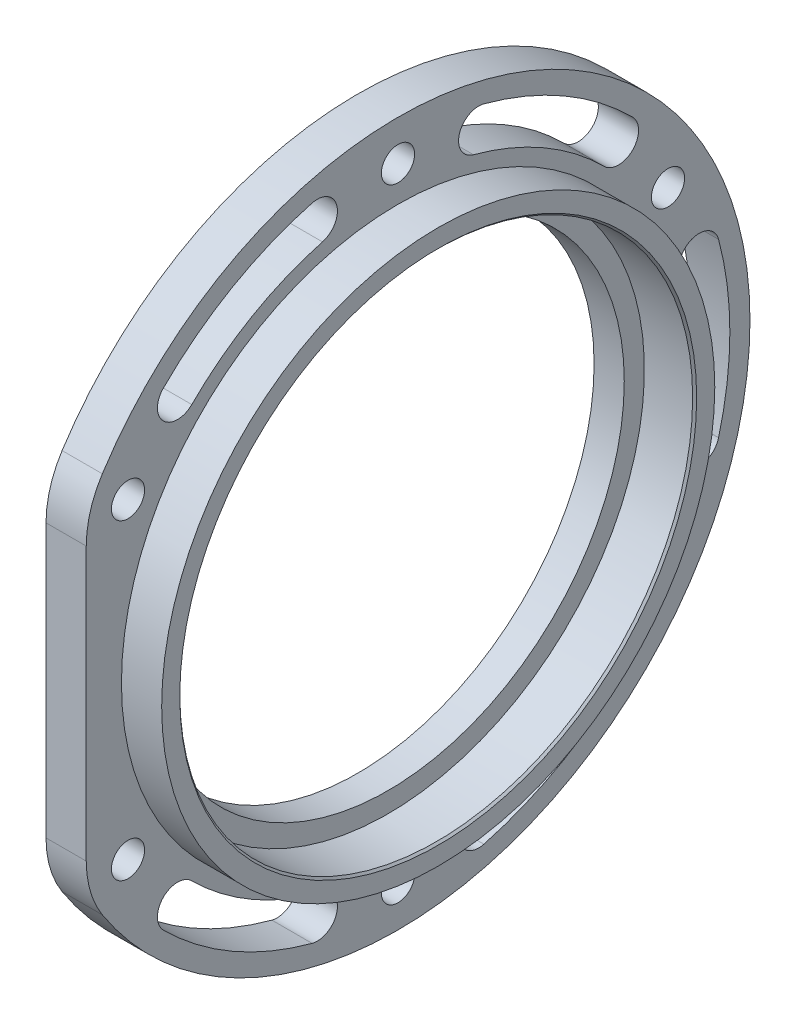
SolidWorks part; units mm, degrees
material "6061 合金"
ref_plane "前视基准面" through (0, 0, 0) normal (0, 0, 1) x (1, 0, 0)
ref_plane "上视基准面" through (0, 0, 0) normal (0, 1, 0) x (1, 0, 0)
ref_plane "右视基准面" through (0, 0, 0) normal (1, 0, 0) x (0, 0, -1)
other "Configuration Table"
sketch "草图1" plane through (0, 0, 0) normal (0, 1, 0) x (1, 0, 0)
  line L0 (-554.3921, 0) -> (27165.2107, 0) construction
  line L1 (0, 23.5) -> (0, 35)
  line L4 (0, 35) -> (4, 35)
  line L6 (8, 25.5) -> (3, 25.5)
  line L7 (3, 25.5) -> (3, 23.5)
  line L8 (3, 23.5) -> (0, 23.5)
  line L9 (4, 35) -> (4, 27.5)
  line L10 (4, 27.5) -> (8, 27.5)
  line L11 (8, 27.5) -> (8, 25.5)
  dimension "D1" = 47
  dimension "D2" = 51
  dimension "D3" = 5
  dimension "D4" = 4
  dimension "D6" = 70
  dimension "D7" = 3
  dimension "D9" = 55
revolve "旋转1" add sketch "草图1" angle 360 about L0
sketch "草图2" plane through (4, 0, 0) normal (1, 0, 0) x (0, 0, -1)
  circle A0 centre (0, 0) radius 31 construction
  point P3 (0, 31)
  point P6 (26.8468, 15.5)
  point P7 (26.8468, -15.5)
  point P8 (0, -31)
  point P9 (-26.8468, -15.5)
  point P10 (-26.8468, 15.5)
  point P11 (0, 0)
  dimension "D1" = 62
  dimension "D2" = 6
hole_wizard "M4 螺纹孔1" positions "草图2" profile "草图3" tap size "M4" standard "ISO" end condition through all
sketch "草图3" plane through (4, 0, 0) normal (0, 1, 0) x (0, 0, -1)
  line L0 (0, 0) -> (0, 4)
  line L1 (0, 4) -> (1.65, 4)
  line L2 (1.65, 4) -> (1.65, 0)
  line L5 (1.65, 0) -> (0, 0)
  line L11 (0, -6.35) -> (0, 107.95) construction
  dimension "通孔螺纹孔钻头直径" = 3.3
  dimension "通孔螺纹孔钻头深度" = 4
cosmetic thread "孔螺纹线1" parameters "D2"=4
cosmetic thread "孔螺纹线2" parameters "D2"=4
cosmetic thread "孔螺纹线3" parameters "D2"=4
cosmetic thread "孔螺纹线4" parameters "D2"=4
cosmetic thread "孔螺纹线5" parameters "D2"=4
cosmetic thread "孔螺纹线6" parameters "D2"=4
sketch "草图4" plane through (4, 0, 0) normal (1, 0, 0) x (0, 0, -1)
  line L0 (-31, -16.2481) -> (-31, 16.2481)
  line L1 (-26.8468, 15.5) -> (-26.8468, -15.5) construction
  circle A0 centre (0, 0) radius 35 construction
  circle A2 centre (0, 0) radius 35
  arc A3 (-31, 16.2481) -> (-31, -16.2481) centre (0, 0) ccw
  dimension "D1" = 31
  dimension "D2" = 0
extrude "切除-拉伸1" cut sketch "草图4" against normal blind 10
fillet "圆角1" radius 10 2 edges at (2, -16.2481, 31) (2, 16.2481, 31)
sketch "草图5" plane through (4, 0, 0) normal (1, 0, 0) x (0, 0, -1)
  line L0 (0, 31) -> (0, 0) construction
  line L1 (0, 0) -> (15.5, 26.8468) construction
  line L2 (8.0234, 29.9437) -> (0, 0) construction
  line L3 (0, 0) -> (21.9203, 21.9203) construction
  arc A0 (8.0234, 29.9437) -> (21.9203, 21.9203) centre (0, 0) cw construction
  arc A1 (23.3345, 23.3345) -> (8.541, 31.8756) centre (0, 0) ccw
  arc A2 (20.5061, 20.5061) -> (7.5058, 28.0118) centre (0, 0) ccw
  arc A3 (20.5061, 20.5061) -> (23.3345, 23.3345) centre (21.9203, 21.9203) ccw
  arc A4 (8.541, 31.8756) -> (7.5058, 28.0118) centre (8.0234, 29.9437) ccw
  arc A5 (29.9437, 8.0234) -> (29.9437, -8.0234) centre (0, 0) cw construction
  arc A6 (31.8756, -8.541) -> (31.8756, 8.541) centre (0, 0) ccw
  arc A7 (28.0118, -7.5058) -> (28.0118, 7.5058) centre (0, 0) ccw
  arc A8 (28.0118, -7.5058) -> (31.8756, -8.541) centre (29.9437, -8.0234) ccw
  arc A9 (31.8756, 8.541) -> (28.0118, 7.5058) centre (29.9437, 8.0234) ccw
  arc A10 (21.9203, -21.9203) -> (8.0234, -29.9437) centre (0, 0) cw construction
  arc A11 (8.541, -31.8756) -> (23.3345, -23.3345) centre (0, 0) ccw
  arc A12 (7.5058, -28.0118) -> (20.5061, -20.5061) centre (0, 0) ccw
  arc A13 (7.5058, -28.0118) -> (8.541, -31.8756) centre (8.0234, -29.9437) ccw
  arc A14 (23.3345, -23.3345) -> (20.5061, -20.5061) centre (21.9203, -21.9203) ccw
  arc A15 (-8.0234, -29.9437) -> (-21.9203, -21.9203) centre (0, 0) cw construction
  arc A16 (-23.3345, -23.3345) -> (-8.541, -31.8756) centre (0, 0) ccw
  arc A17 (-20.5061, -20.5061) -> (-7.5058, -28.0118) centre (0, 0) ccw
  arc A18 (-20.5061, -20.5061) -> (-23.3345, -23.3345) centre (-21.9203, -21.9203) ccw
  arc A19 (-8.541, -31.8756) -> (-7.5058, -28.0118) centre (-8.0234, -29.9437) ccw
  arc A25 (-21.9203, 21.9203) -> (-8.0234, 29.9437) centre (0, 0) cw construction
  arc A26 (-8.541, 31.8756) -> (-23.3345, 23.3345) centre (0, 0) ccw
  arc A27 (-7.5058, 28.0118) -> (-20.5061, 20.5061) centre (0, 0) ccw
  arc A28 (-7.5058, 28.0118) -> (-8.541, 31.8756) centre (-8.0234, 29.9437) ccw
  arc A29 (-23.3345, 23.3345) -> (-20.5061, 20.5061) centre (-21.9203, 21.9203) ccw
  arc A40 (-29.9437, -8.0234) -> (-29.9437, 8.0234) centre (0, 0) cw construction
  arc A41 (-31.8756, 8.541) -> (-31.8756, -8.541) centre (0, 0) ccw
  arc A42 (-28.0118, 7.5058) -> (-28.0118, -7.5058) centre (0, 0) ccw
  arc A43 (-28.0118, 7.5058) -> (-31.8756, 8.541) centre (-29.9437, 8.0234) ccw
  arc A44 (-31.8756, -8.541) -> (-28.0118, -7.5058) centre (-29.9437, -8.0234) ccw
  point P4 (15.5, 26.8468)
  point P19 (31, 0)
  point P26 (15.5, -26.8468)
  point P33 (-15.5, -26.8468)
  point P47 (-15.5, 26.8468)
  point P52 (0, 0)
  point P54 (-31, 0)
  point P62 (-31, 0)
  point P70 (-31, 0)
  dimension "D1" = 30
  dimension "D3" = 4
  dimension "D4" = 31
  dimension "D2" = 30
  dimension "D5" = 6
extrude "切除-拉伸2" cut sketch "草图5" against normal blind 10
chamfer "倒角1" distance 0.2 angle 45 1 edges at (8, 0, 25.5)
